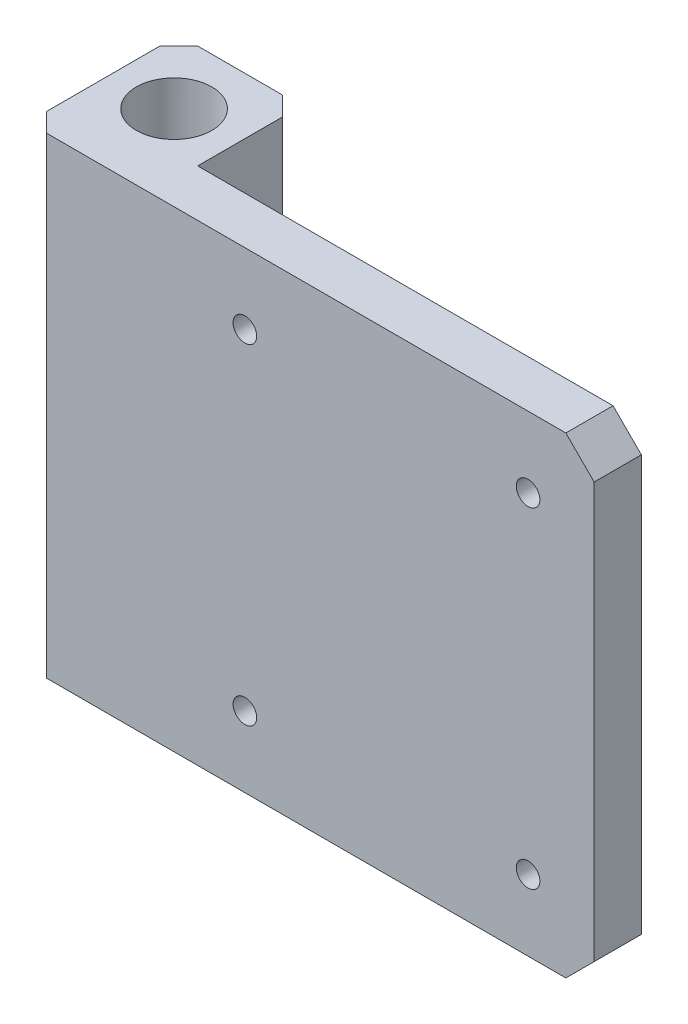
from build123d import *

# Parameters (mm, degrees)
BOSS_EXTRUDE1_DEPTH   = 50
SKETCH2_R             = 0.75
CUT_EXTRUDE1_DEPTH    = 10
SKETCH3_R             = 4
CUT_EXTRUDE2_DEPTH    = 60
CHAMFER1_SIZE         = 2
LPATTERN1_COUNT       = 2
LPATTERN1_PITCH       = 30
CHAMFER2_SIZE         = 3
M3_TAPPED_HOLE1_D     = 2.5
M3_TAPPED_HOLE1_DEPTH = 7.5
M3_TAPPED_HOLE1_TIP   = 0.751075774
CHAMFER3_SIZE         = 0.8


with BuildPart() as part:
    # Sketch1 → Boss-Extrude1 (new body)
    with BuildSketch(Plane(origin=(0, 0, 0), x_dir=(1, 0, 0), z_dir=(0, 1, 0))):
        Polygon((0, 0), (60, 0), (60, 5), (13, 5), (13, 16), (0, 16), align=None)
    extrude(amount=BOSS_EXTRUDE1_DEPTH)

    # Sketch2 → Cut-Extrude1 (cut)
    with BuildSketch(Plane.XY):
        with Locations((53, 42.5)):
            Circle(SKETCH2_R)
        with Locations((53, 7.5)):
            Circle(SKETCH2_R)
    cut_extrude1 = extrude(amount=-CUT_EXTRUDE1_DEPTH, mode=Mode.SUBTRACT)

    # Sketch3 → Cut-Extrude2 (cut)
    with BuildSketch(Plane(origin=(0, 50, 0), x_dir=(1, 0, 0), z_dir=(0, 1, 0))):
        with Locations(Location((6.5, 9, 0), (0, 0, 270))):
            Circle(SKETCH3_R)
    extrude(amount=-CUT_EXTRUDE2_DEPTH, mode=Mode.SUBTRACT)

    # Chamfer1
    chamfer1_edges = [part.edges().sort_by_distance(p)[0] for p in [
        (0, 25, -16),
        (13, 25, -16),
        (0, 25, 0),
    ]]
    chamfer(chamfer1_edges, length=CHAMFER1_SIZE)

    # LPattern1: Cut-Extrude1 ×2
    with Locations(*[(-i * LPATTERN1_PITCH, 0, 0) for i in range(1, LPATTERN1_COUNT)]):
        add(cut_extrude1, mode=Mode.SUBTRACT)

    # Chamfer2
    chamfer2_edges = [part.edges().sort_by_distance(p)[0] for p in [
        (60, 50, -2.5),
        (60, 0, -2.5),
    ]]
    chamfer(chamfer2_edges, length=CHAMFER2_SIZE)

    # M3 Tapped Hole1
    with Locations(Plane(origin=(23, 42.5, 0), x_dir=(1, 0, 0), z_dir=(0, 0, 1))):
        with Locations((0, 0), (30, 0), (30, -35), (0, -35)):
            Hole(M3_TAPPED_HOLE1_D / 2, depth=M3_TAPPED_HOLE1_DEPTH)
            with Locations((0, 0, -(M3_TAPPED_HOLE1_DEPTH + M3_TAPPED_HOLE1_TIP / 2))):  # 118° drill point
                Cone(0, M3_TAPPED_HOLE1_D / 2, M3_TAPPED_HOLE1_TIP, mode=Mode.SUBTRACT)

    # Chamfer3
    chamfer3_edges = [part.edges().sort_by_distance(p)[0] for p in [
        (24.25, 7.5, -5),
        (54.25, 7.5, -5),
        (54.25, 42.5, -5),
        (24.25, 42.5, -5),
    ]]
    chamfer(chamfer3_edges, length=CHAMFER3_SIZE)


solid = part.part
